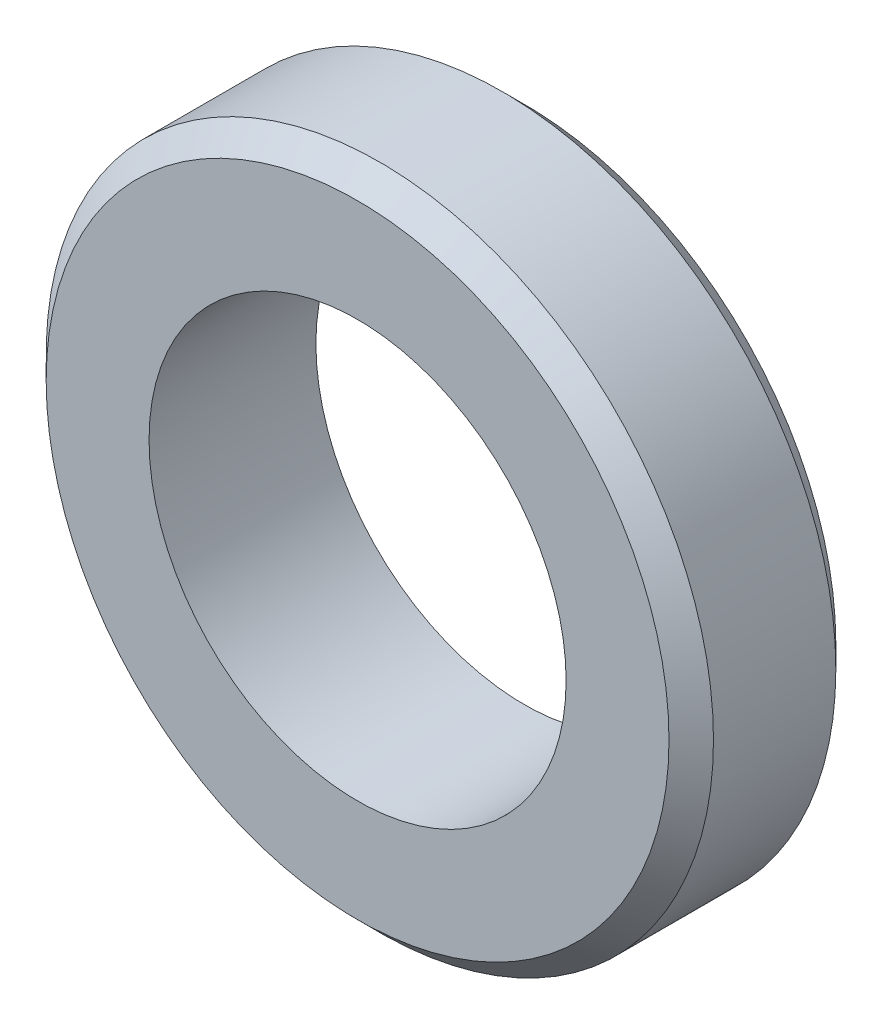
from build123d import *

# Parameters (mm, degrees)
SKETCH1_R              = 30
BOSS_EXTRUDE1_DEPTH    = 15
SKETCH2_R              = 17.5
CUT_EXTRUDE1_DEPTH     = 15
CHAMFER1_SIZE          = 2
M42_TAPPED_HOLE4_D     = 37.5
M42_TAPPED_HOLE4_DEPTH = 106.5
M42_TAPPED_HOLE4_TIP   = 11.266136607


with BuildPart() as part:
    # Sketch1 → Boss-Extrude1 (new body)
    with BuildSketch(Plane.XY):
        Circle(SKETCH1_R)
    extrude(amount=BOSS_EXTRUDE1_DEPTH)

    # Sketch2 → Cut-Extrude1 (cut)
    with BuildSketch(Plane.XY.offset(15)):
        Circle(SKETCH2_R)
    extrude(amount=-CUT_EXTRUDE1_DEPTH, mode=Mode.SUBTRACT)

    # Chamfer1
    chamfer1_edges = [part.edges().sort_by_distance(p)[0] for p in [
        (-30, 0, 0),
        (-30, 0, 15),
    ]]
    chamfer(chamfer1_edges, length=CHAMFER1_SIZE)

    # M42 Tapped Hole4
    with Locations(Plane.XY.offset(15)):
        with Locations((0, 0)):
            Hole(M42_TAPPED_HOLE4_D / 2, depth=M42_TAPPED_HOLE4_DEPTH)
            with Locations((0, 0, -(M42_TAPPED_HOLE4_DEPTH + M42_TAPPED_HOLE4_TIP / 2))):  # 118° drill point
                Cone(0, M42_TAPPED_HOLE4_D / 2, M42_TAPPED_HOLE4_TIP, mode=Mode.SUBTRACT)


solid = part.part
